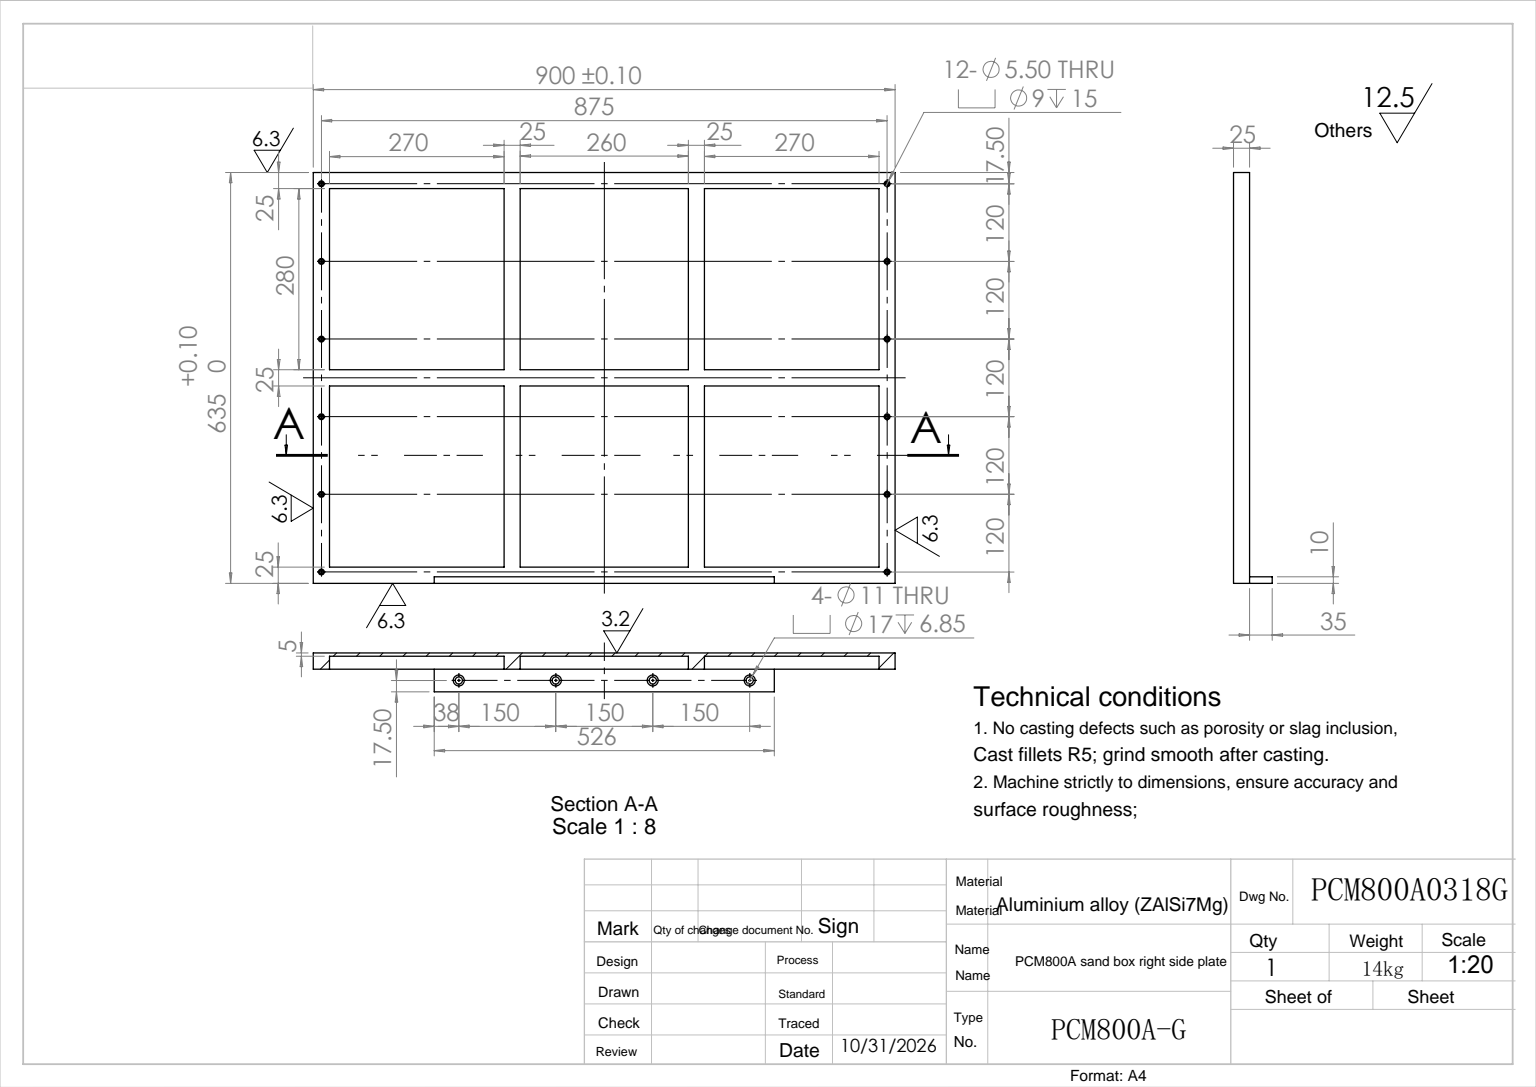
SolidWorks part; units mm, degrees
ref_plane "前视" through (0, 0, 0) normal (0, 0, 1) x (1, 0, 0)
ref_plane "上视" through (0, 0, 0) normal (0, 1, 0) x (1, 0, 0)
ref_plane "右视" through (0, 0, 0) normal (1, 0, 0) x (0, 0, -1)
sketch "草图1" plane through (0, 0, 0) normal (1, 0, 0) x (0, 0, -1)
  line L1 (0, 0) -> (900, 0)
  line L2 (0, 0) -> (0, 635)
  line L3 (0, 635) -> (900, 635)
  line L4 (900, 0) -> (900, 635)
  dimension "D1" = 635
  dimension "D2" = 900
extrude "拉伸1" add sketch "草图1" along normal blind 5
sketch "草图2" plane through (5, 0, 0) normal (1, 0, 0) x (0, 0, -1)
  line L1 (0, 0) -> (900, 0) construction
  line L2 (0, 635) -> (25, 635)
  line L3 (0, 635) -> (0, 0)
  line L4 (0, 0) -> (25, 0)
  line L7 (25, 635) -> (25, 0)
  line L9 (900, 635) -> (875, 635)
  line L10 (900, 635) -> (900, 0)
  line L11 (900, 0) -> (875, 0)
  line L12 (875, 635) -> (875, 0)
  dimension "D1" = 25
  dimension "D2" = 25
extrude "拉伸2" add sketch "草图2" along normal blind 20
sketch "草图4" plane through (5, 0, 0) normal (1, 0, 0) x (0, 0, -1)
  line L0 (875, 635) -> (875, 0) construction
  line L1 (25, 635) -> (875, 635)
  line L2 (25, 635) -> (25, 610)
  line L3 (25, 610) -> (875, 610)
  line L4 (875, 635) -> (875, 610)
  line L5 (875, 635) -> (875, 0) construction
  line L6 (25, 0) -> (875, 0)
  line L7 (25, 0) -> (25, 25)
  line L8 (25, 25) -> (875, 25)
  line L9 (875, 0) -> (875, 25)
  dimension "D1" = 25
  dimension "D2" = 25
extrude "拉伸3" add sketch "草图4" along normal blind 20
sketch "草图5" plane through (5, 0, 0) normal (1, 0, 0) x (0, 0, -1)
  line L0 (25, 610) -> (875, 610) construction
  line L1 (295, 610) -> (320, 610)
  line L2 (295, 610) -> (295, 25)
  line L3 (295, 25) -> (320, 25)
  line L4 (320, 610) -> (320, 25)
  line L5 (875, 25) -> (25, 25) construction
  line L6 (25, 610) -> (875, 610) construction
  line L7 (580, 610) -> (605, 610)
  line L8 (580, 610) -> (580, 25)
  line L9 (580, 25) -> (605, 25)
  line L10 (605, 610) -> (605, 25)
  line L11 (25, 25) -> (25, 610) construction
  line L12 (875, 610) -> (875, 25) construction
  dimension "D1" = 25
  dimension "D2" = 25
  dimension "D3" = 270
  dimension "D4" = 270
extrude "拉伸4" add sketch "草图5" along normal blind 20
sketch "草图6" plane through (5, 0, 0) normal (1, 0, 0) x (0, 0, -1)
  line L0 (25, 25) -> (25, 610) construction
  line L1 (25, 330) -> (875, 330)
  line L2 (25, 330) -> (25, 305)
  line L3 (25, 305) -> (875, 305)
  line L4 (875, 330) -> (875, 305)
  line L5 (875, 610) -> (875, 25) construction
  line L6 (295, 25) -> (25, 25) construction
  dimension "D1" = 25
  dimension "D2" = 280
extrude "拉伸5" add sketch "草图6" along normal blind 20
sketch "草图7" plane through (25, 0, 0) normal (1, 0, 0) x (0, 0, -1)
  line L0 (0, 0) -> (900, 0) construction
  line L1 (187, 0) -> (713, 0)
  line L2 (187, 0) -> (187, 10)
  line L3 (187, 10) -> (713, 10)
  line L4 (713, 0) -> (713, 10)
  line L5 (900, 0) -> (900, 635) construction
  dimension "D1" = 10
  dimension "D2" = 526
  dimension "D3" = 187
extrude "拉伸6" add sketch "草图7" along normal blind 35
sketch "草图24" plane through (0, 10, 0) normal (0, 1, 0) x (-1, 0, 0)
  line L0 (-42.5, -713) -> (-42.5, -187) construction
  line L1 (-60, -713) -> (-25, -713) construction
  line L2 (-60, -187) -> (-25, -187) construction
  line L3 (-42.5, -675) -> (-60, -675) construction
  line L4 (-60, -713) -> (-60, -187) construction
  line L5 (-42.5, -525) -> (-60, -525) construction
  line L6 (-42.5, -375) -> (-60, -375) construction
  line L7 (-42.5, -225) -> (-60, -225) construction
  dimension "D1" = 38
  dimension "D2" = 150
  dimension "D3" = 150
  dimension "D4" = 150
hole_wizard "孔1" positions "3D草图9" profile "草图25" legacy end condition through all
sketch3d "3D草图9"
  point P0 (42.5, 10, -675)
  point P3 (42.5, 10, -525)
  point P6 (42.5, 10, -375)
  point P9 (42.5, 10, -225)
sketch "草图25" plane through (42.5, 10, -675) normal (1, 0, 0) x (0, 0, 1)
  line L0 (0, 0) -> (0, 10)
  line L1 (0, 10) -> (5.5, 10)
  line L3 (5.5, 10) -> (5.5, 6.85)
  line L4 (5.5, 6.85) -> (8.5, 6.85)
  line L5 (8.5, 6.85) -> (8.5, 0)
  line L7 (8.5, 0) -> (0, 0)
  line L11 (0, -6.35) -> (0, 107.95) construction
  dimension "籵謂謂眻噤" = 11
  dimension "籵謂謂旮僅" = 10
  dimension "翐倛麥芛謂眻噤" = 17
  dimension "翐倛麥芛謂旮僅" = 6.85
sketch "草图26" plane through (25, 0, 0) normal (1, 0, 0) x (0, 0, -1)
  line L0 (12.5, 635) -> (12.5, 0) construction
  line L1 (900, 635) -> (0, 635) construction
  line L2 (0, 0) -> (187, 0) construction
  line L5 (0, 635) -> (0, 0) construction
  line L7 (12.5, 617.5) -> (0, 617.5) construction
  line L8 (12.5, 497.5) -> (0, 497.5) construction
  line L9 (12.5, 377.5) -> (0, 377.5) construction
  line L10 (12.5, 257.5) -> (0, 257.5) construction
  line L11 (12.5, 137.5) -> (0, 137.5) construction
  line L12 (12.5, 17.5) -> (0, 17.5) construction
  dimension "D1" = 12.5
  dimension "D3" = 17.5
  dimension "D4" = 120
  dimension "D5" = 120
  dimension "D6" = 120
  dimension "D7" = 120
  dimension "D8" = 120
hole_wizard "孔2" positions "3D草图10" profile "草图27" legacy end condition through all
sketch3d "3D草图10"
  point P0 (25, 617.5, -12.5)
  point P3 (25, 497.5, -12.5)
  point P6 (25, 377.5, -12.5)
  point P9 (25, 257.5, -12.5)
  point P12 (25, 137.5, -12.5)
  point P15 (25, 17.5, -12.5)
sketch "草图27" plane through (25, 617.5, -12.5) normal (0, 1, 0) x (0, 0, -1)
  line L0 (0, 0) -> (0, 25)
  line L1 (0, 25) -> (2.75, 25)
  line L3 (2.75, 25) -> (2.75, 15)
  line L4 (2.75, 15) -> (4.5, 15)
  line L5 (4.5, 15) -> (4.5, 0)
  line L7 (4.5, 0) -> (0, 0)
  line L11 (0, -6.35) -> (0, 107.95) construction
  dimension "籵謂謂眻噤" = 5.5
  dimension "籵謂謂旮僅" = 25
  dimension "翐倛麥芛謂眻噤" = 9
  dimension "翐倛麥芛謂旮僅" = 15
ref_plane "基准面1" through (0, 0, -450) normal (0, 0, 1) x (1, 0, 0)
mirror "镜向1" about plane through (0, 0, -450) normal (0, 0, 1) of "孔2"
